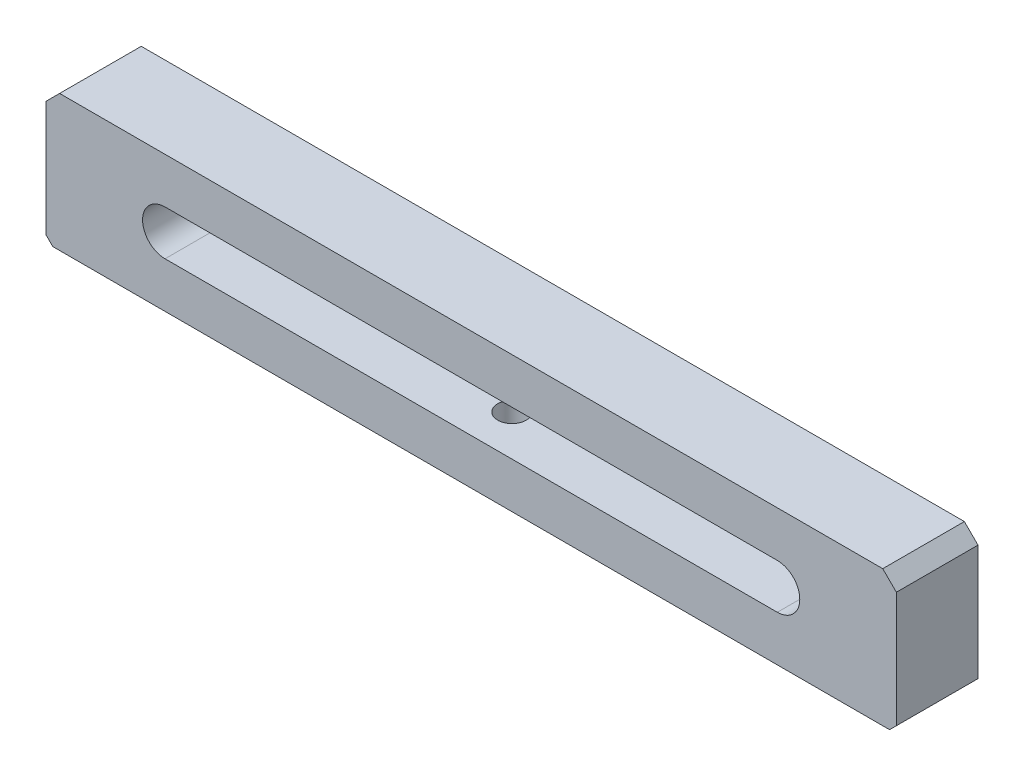
from build123d import *

# Parameters (mm, degrees)
SKETCH_1_W             = 125
SKETCH_1_H             = 20
EXTRUDE_1_DEPTH        = 12
CUT_EXTRUDE_1_DEPTH    = 65.422433981
HOLE_WIZARD_M5_1_D     = 4.2
HOLE_WIZARD_M5_1_DEPTH = 10
HOLE_WIZARD_M5_1_TIP   = 1.2618073
CHAMFER_1_SIZE         = 2
CHAMFER_2_SIZE         = 1


with BuildPart() as part:
    # 草图1 → 凸台-拉伸1 (new body)
    with BuildSketch(Plane.XY):
        Rectangle(SKETCH_1_W, SKETCH_1_H)
    extrude(amount=EXTRUDE_1_DEPTH)

    # 草图2 → 切除-拉伸1 (cut, through all)
    with BuildSketch(Plane.XY.offset(12)):
        with BuildLine():
            Line((-45, 3.3), (45, 3.3))
            ThreePointArc((45, 3.3), (48.3, 0), (45, -3.3))
            Line((45, -3.3), (-45, -3.3))
            ThreePointArc((-45, -3.3), (-48.3, 0), (-45, 3.3))
        make_face()
    extrude(amount=-CUT_EXTRUDE_1_DEPTH, mode=Mode.SUBTRACT)

    # M5 螺纹孔1
    with Locations(Plane(origin=(0, -10, 0), x_dir=(-1, 0, 0), z_dir=(0, -1, 0))):
        with Locations((55, -6), (0, -6), (-55, -6)):
            Hole(HOLE_WIZARD_M5_1_D / 2, depth=HOLE_WIZARD_M5_1_DEPTH)
            with Locations((0, 0, -(HOLE_WIZARD_M5_1_DEPTH + HOLE_WIZARD_M5_1_TIP / 2))):  # 118° drill point
                Cone(0, HOLE_WIZARD_M5_1_D / 2, HOLE_WIZARD_M5_1_TIP, mode=Mode.SUBTRACT)

    # 倒角1
    chamfer_1_edges = [part.edges().sort_by_distance(p)[0] for p in [
        (-62.5, 10, 6),
        (62.5, 10, 6),
    ]]
    chamfer(chamfer_1_edges, length=CHAMFER_1_SIZE)

    # 倒角2
    chamfer_2_edges = [part.edges().sort_by_distance(p)[0] for p in [
        (62.5, -10, 6),
        (-62.5, -10, 6),
    ]]
    chamfer(chamfer_2_edges, length=CHAMFER_2_SIZE)


solid = part.part
